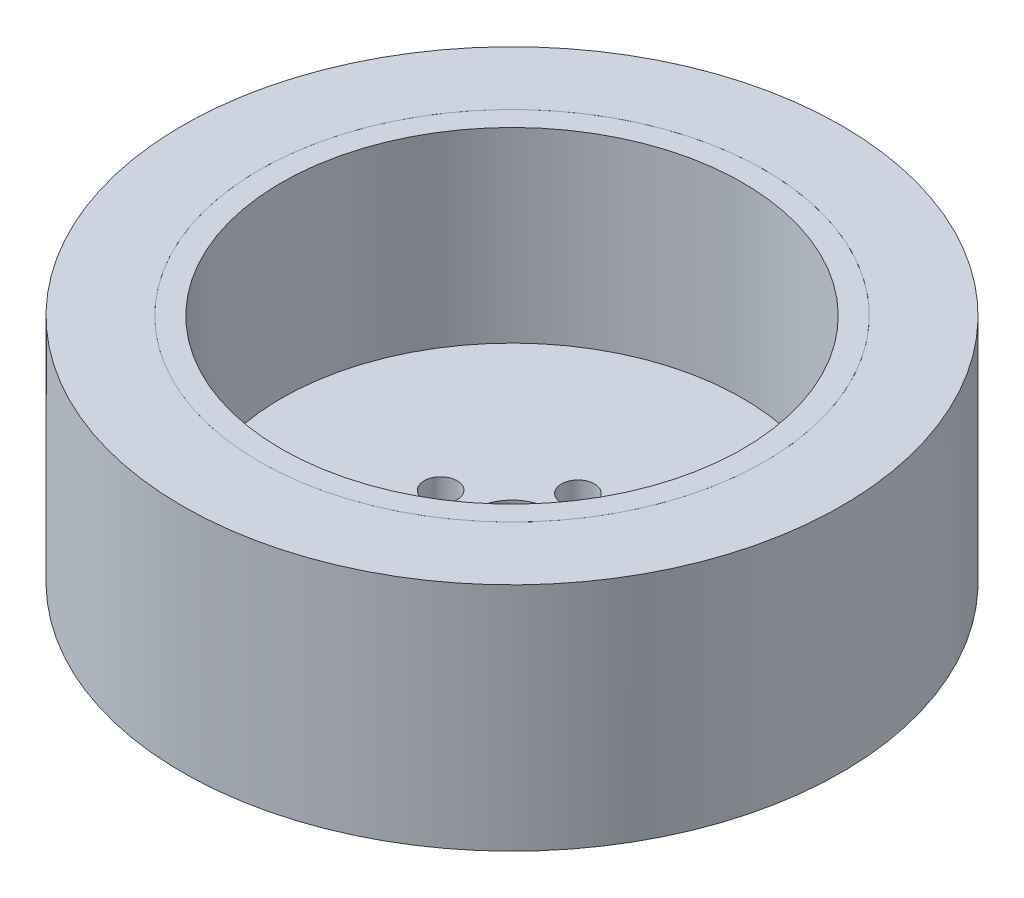
from build123d import *

# Parameters (mm, degrees)
SKETCH_1_R      = 23
SKETCH_1_R_2    = 1.5
SKETCH_1_R_3    = 3.5
EXTRUDE_1_DEPTH = 4
SKETCH_2_R      = 23
SKETCH_2_R_2    = 21
EXTRUDE_2_DEPTH = 17
SKETCH_3_R      = 30
SKETCH_3_R_2    = 23
EXTRUDE_3_DEPTH = 21


with BuildPart() as part:
    # 草图1 → 凸台-拉伸1 (new body)
    with BuildSketch(Plane(origin=(0, 0, 0), x_dir=(1, 0, 0), z_dir=(0, 1, 0))):
        with Locations(Location((0, 0, 0), (0, 0, 270))):
            Circle(SKETCH_1_R)
        with Locations(Location((6.5, 0, 0), (0, 0, 270))):
            Circle(SKETCH_1_R_2, mode=Mode.SUBTRACT)
        with Locations(Location((-6.5, 0, 0), (0, 0, 270))):
            Circle(SKETCH_1_R_2, mode=Mode.SUBTRACT)
        with Locations(Location((0, -6, 0), (0, 0, 270))):
            Circle(SKETCH_1_R_2, mode=Mode.SUBTRACT)
        with Locations(Location((0, 6, 0), (0, 0, 270))):
            Circle(SKETCH_1_R_2, mode=Mode.SUBTRACT)
        with Locations(Location((0, 0, 0), (0, 0, 270))):
            Circle(SKETCH_1_R_3, mode=Mode.SUBTRACT)
    extrude(amount=EXTRUDE_1_DEPTH)

    # 草图2 → 凸台-拉伸2 (add)
    with BuildSketch(Plane(origin=(0, 4, 0), x_dir=(1, 0, 0), z_dir=(0, 1, 0))):
        with Locations(Location((0, 0, 0), (0, 0, 270))):
            Circle(SKETCH_2_R)
        with Locations(Location((0, 0, 0), (0, 0, 270))):
            Circle(SKETCH_2_R_2, mode=Mode.SUBTRACT)
    extrude(amount=EXTRUDE_2_DEPTH)


with BuildPart() as body_2:
    # 草图3 → 凸台-拉伸3 (new body)
    with BuildSketch(Plane.XZ):
        with Locations(Location((0, 0, 0), (0, 0, 270))):
            Circle(SKETCH_3_R)
        with Locations(Location((0, 0, 0), (0, 0, 270))):
            Circle(SKETCH_3_R_2, mode=Mode.SUBTRACT)
    extrude(amount=-EXTRUDE_3_DEPTH)


solid = Compound([part.part, body_2.part])
